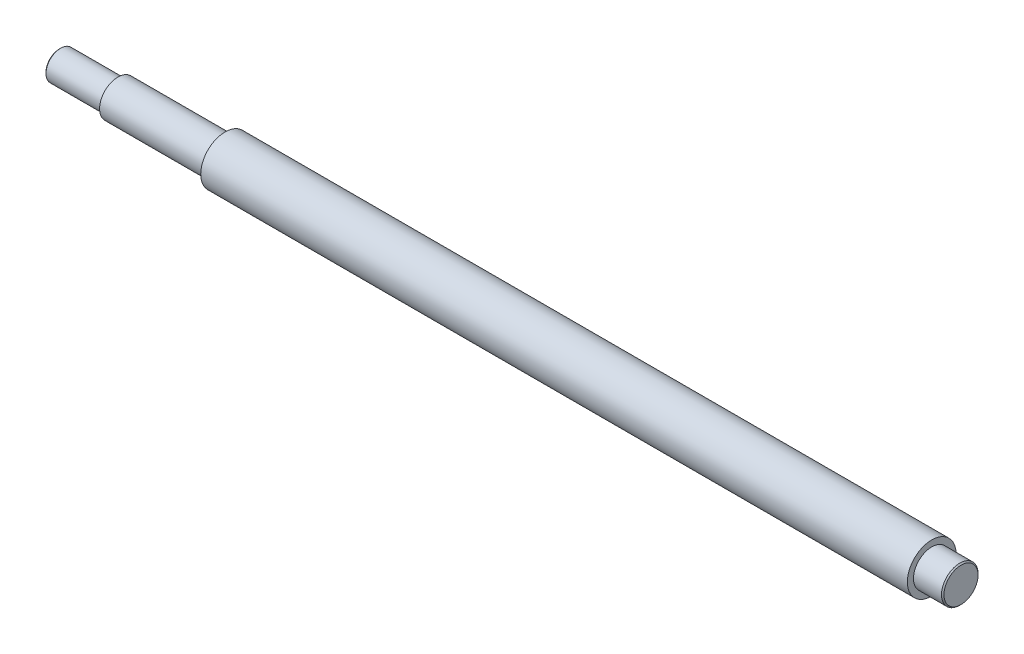
from build123d import *

# Parameters (mm, degrees)
CUT_EXTRUDE_1_DEPTH = 2.2
CHAMFER_1_SIZE      = 0.5


with BuildPart() as part:
    # 草图1 → 旋转1 (revolve)
    with BuildSketch(Plane(origin=(0, 0, 0), x_dir=(1, 0, 0), z_dir=(0, 1, 0)), mode=Mode.PRIVATE) as revolve_1_sk:
        Polygon((0, 0), (0, 6), (24, 6), (24, 7.5), (68, 7.5), (68, 10), (358, 10), (358, 7.5), (370, 7.5), (370, 0), align=None)
    revolve(revolve_1_sk.sketch.rotate(Axis((0, 0, 0), (1, 0, 0)), 180), axis=Axis((0, 0, 0), (1, 0, 0)))

    # 草图2 → 切除-拉伸1 (cut)
    with BuildSketch(Plane(origin=(0, -6, 0), x_dir=(-1, 0, 0), z_dir=(0, -1, 0))):
        with BuildLine():
            Line((-21, 2), (-3, 2))
            ThreePointArc((-3, 2), (-1, 0), (-3, -2))
            Line((-3, -2), (-21, -2))
            ThreePointArc((-21, -2), (-23, 0), (-21, 2))
        make_face()
    extrude(amount=-CUT_EXTRUDE_1_DEPTH, mode=Mode.SUBTRACT)

    # 倒角1
    chamfer_1_edges = [part.edges().sort_by_distance(p)[0] for p in [
        (0, 0, -6),
        (370, 0, -7.5),
    ]]
    chamfer(chamfer_1_edges, length=CHAMFER_1_SIZE)


solid = part.part
